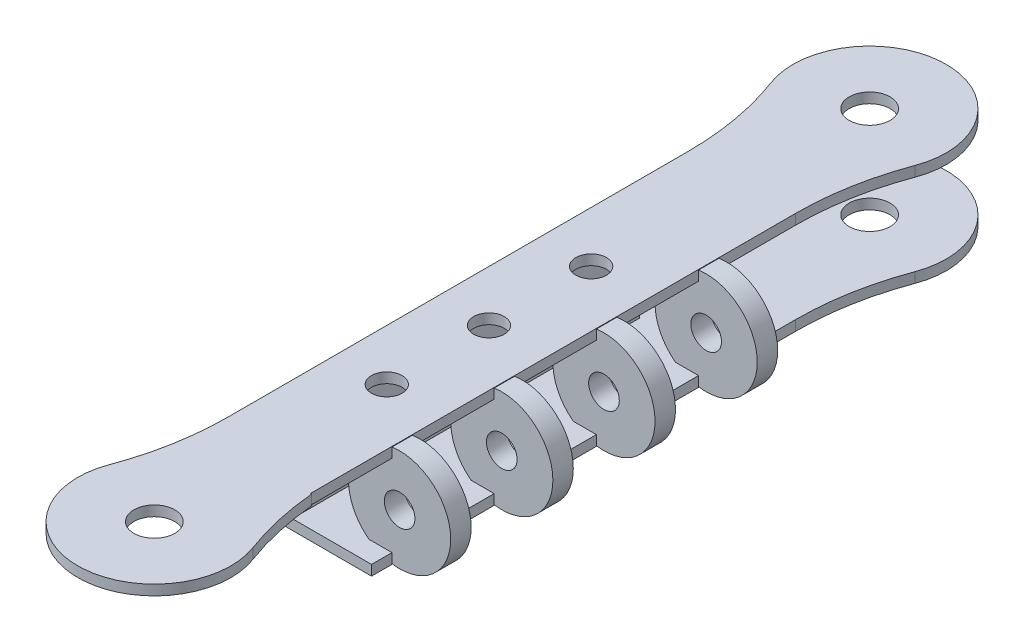
from build123d import *

# Parameters (mm, degrees)
BOSS_EXTRUDE1_DEPTH     = 10
CUT_EXTRUDE1_DEPTH      = 79.501592341
CUT_EXTRUDE1_DEPTH_BACK = 79.501592341
SKETCH2_R               = 2
CUT_EXTRUDE4_DEPTH      = 79.501592341
CUT_EXTRUDE4_DEPTH_BACK = 79.501592341
SKETCH5_W               = 10
SKETCH5_H               = 8
SKETCH3_R               = 5
BOSS_EXTRUDE2_DEPTH     = 40
CUT_EXTRUDE3_DEPTH      = 79.912926724
CUT_EXTRUDE3_DEPTH_BACK = 79.912926724
SKETCH4_W               = 4
SKETCH4_H               = 8
CUT_EXTRUDE5_DEPTH      = 80.176595509
CUT_EXTRUDE5_DEPTH_BACK = 5
SKETCH6_W               = 8
SKETCH6_H               = 7.999190419
SKETCH6_H_2             = 8
SKETCH6_H_3             = 8.000809581
SKETCH6_H_4             = 8.001619162
SKETCH7_W               = 5
SKETCH7_H               = 8
CUT_EXTRUDE6_DEPTH      = 60.390655831
CUT_EXTRUDE8_DEPTH      = 79.912926698
CUT_EXTRUDE8_DEPTH_BACK = 79.912926698
SKETCH9_R               = 1.5
CUT_EXTRUDE9_DEPTH      = 62.329030646
CUT_EXTRUDE9_DEPTH_BACK = 62.329030646
SKETCH10_R              = 1.5
SKETCH11_W              = 18
SKETCH11_H              = 9
CUT_EXTRUDE10_DEPTH     = 70.117653317
CUT_EXTRUDE11_DEPTH     = 6


with BuildPart() as part:
    # Sketch1 → Boss-Extrude1 (new body)
    with BuildSketch(Plane(origin=(0, 0, 0), x_dir=(1, 0, 0), z_dir=(0, 1, 0))):
        with BuildLine():
            Line((-5.254735448, -12.5), (-5.254735448, -57.5))
            ThreePointArc((-5.254735448, -57.5), (-5.702369539, -62.524085228), (-7.031169787, -67.389894366))
            ThreePointArc((-7.031169787, -67.389894366), (-7.381862008, -68.674061352), (-7.5, -70))
            ThreePointArc((-7.5, -70), (0, -77.5), (7.5, -70))
            ThreePointArc((7.5, -70), (7.381862008, -68.674061352), (7.031169787, -67.389894366))
            ThreePointArc((7.031169787, -67.389894366), (5.702369539, -62.524085228), (5.254735448, -57.5))
            Line((5.254735448, -57.5), (5.254735448, -12.5))
            ThreePointArc((5.254735448, -12.5), (5.702369539, -7.475914772), (7.031169787, -2.610105634))
            ThreePointArc((7.031169787, -2.610105634), (7.381862008, -1.325938648), (7.5, 0))
            ThreePointArc((7.5, 0), (0, 7.5), (-7.5, 0))
            ThreePointArc((-7.5, 0), (-7.381862008, -1.325938648), (-7.031169787, -2.610105634))
            ThreePointArc((-7.031169787, -2.610105634), (-5.702369539, -7.475914772), (-5.254735448, -12.5))
        make_face()
    extrude(amount=BOSS_EXTRUDE1_DEPTH)

    # Sketch2 → Cut-Extrude1 (cut, two sides: drawn at the far end of the back side and taken through both)
    with BuildSketch(Plane(origin=(0, 10, 0), x_dir=(1, 0, 0), z_dir=(0, 1, 0)).offset(-CUT_EXTRUDE1_DEPTH_BACK)):
        with Locations(Location((0, 0, 0), (0, 0, 270))):
            Circle(SKETCH2_R)
        with Locations(Location((0, -70, 0), (0, 0, 270))):
            Circle(SKETCH2_R)
    extrude(amount=CUT_EXTRUDE1_DEPTH + CUT_EXTRUDE1_DEPTH_BACK, mode=Mode.SUBTRACT)

    # Sketch5 → Cut-Extrude4 (cut, two sides: drawn at the far end of the back side and taken through both)
    with BuildSketch(Plane.XY.offset(-CUT_EXTRUDE4_DEPTH_BACK)):
        with Locations((2.5, 5)):
            Rectangle(SKETCH5_W, SKETCH5_H)
    extrude(amount=CUT_EXTRUDE4_DEPTH + CUT_EXTRUDE4_DEPTH_BACK, mode=Mode.SUBTRACT)

    # Sketch3 → Boss-Extrude2 (add)
    with BuildSketch(Plane.XY.offset(20)):
        with Locations((6, 5)):
            Circle(SKETCH3_R)
    extrude(amount=BOSS_EXTRUDE2_DEPTH)

    # Sketch4 → Cut-Extrude3 (cut, two sides: drawn at the far end of the back side and taken through both)
    with BuildSketch(Plane(origin=(0, 0, 0), x_dir=(1, 0, 0), z_dir=(0, 1, 0)).offset(-CUT_EXTRUDE3_DEPTH_BACK)):
        with Locations((7.254735448, -26)):
            Rectangle(SKETCH4_W, SKETCH4_H)
        with Locations((7.254735448, -36)):
            Rectangle(SKETCH4_W, SKETCH4_H)
        with Locations((7.254735448, -46)):
            Rectangle(SKETCH4_W, SKETCH4_H)
        with Locations((7.254735448, -56)):
            Rectangle(SKETCH4_W, SKETCH4_H)
    extrude(amount=CUT_EXTRUDE3_DEPTH + CUT_EXTRUDE3_DEPTH_BACK, mode=Mode.SUBTRACT)

    # Sketch6 → Cut-Extrude5 (cut, two sides: drawn at the far end of the back side and taken through both)
    with BuildSketch(Plane(origin=(5.254735448, 0, 0), x_dir=(0, 0, -1), z_dir=(1, 0, 0)).offset(-CUT_EXTRUDE5_DEPTH_BACK)):
        with Locations((-56, 4.99959521)):
            Rectangle(SKETCH6_W, SKETCH6_H)
        with Locations((-46, 5)):
            Rectangle(SKETCH6_W, SKETCH6_H_2)
        with Locations((-36, 5.000404791)):
            Rectangle(SKETCH6_W, SKETCH6_H_3)
        with Locations((-26, 5.000809581)):
            Rectangle(SKETCH6_W, SKETCH6_H_4)
    extrude(amount=CUT_EXTRUDE5_DEPTH + CUT_EXTRUDE5_DEPTH_BACK, mode=Mode.SUBTRACT)

    # Sketch7 → Cut-Extrude6 (cut, through all)
    with BuildSketch(Plane.XY.offset(20)):
        with Locations((-5, 5)):
            Rectangle(SKETCH7_W, SKETCH7_H)
    extrude(amount=-CUT_EXTRUDE6_DEPTH, mode=Mode.SUBTRACT)

    # Sketch9 → Cut-Extrude8 (cut, two sides: drawn at the far end of the back side and taken through both)
    with BuildSketch(Plane(origin=(0, 10, 0), x_dir=(1, 0, 0), z_dir=(0, 1, 0)).offset(-CUT_EXTRUDE8_DEPTH_BACK)):
        with Locations(Location((-0.254735448, -27, 0), (0, 0, 270))):
            Circle(SKETCH9_R)
        with Locations(Location((-0.254735448, -37, 0), (0, 0, 270))):
            Circle(SKETCH9_R)
        with Locations(Location((-0.254735448, -47, 0), (0, 0, 270))):
            Circle(SKETCH9_R)
    extrude(amount=CUT_EXTRUDE8_DEPTH + CUT_EXTRUDE8_DEPTH_BACK, mode=Mode.SUBTRACT)

    # Sketch10 → Cut-Extrude9 (cut, two sides: drawn at the far end of the back side and taken through both)
    with BuildSketch(Plane.XY.offset(52).offset(-CUT_EXTRUDE9_DEPTH_BACK)):
        with Locations((6, 5)):
            Circle(SKETCH10_R)
    extrude(amount=CUT_EXTRUDE9_DEPTH + CUT_EXTRUDE9_DEPTH_BACK, mode=Mode.SUBTRACT)

    # Sketch11 → Cut-Extrude10 (cut, through all)
    with BuildSketch(Plane.XY.offset(60)):
        with Locations((-0.335498684, 4.5)):
            Rectangle(SKETCH11_W, SKETCH11_H)
    extrude(amount=CUT_EXTRUDE10_DEPTH, mode=Mode.SUBTRACT)

    # Sketch12 → Cut-Extrude11 (cut)
    with BuildSketch(Plane.XY.offset(60)):
        Polygon((5.254735448, 0), (5.254735448, 1), (-2.5, 1), (-2.5, 9), (-5.364914213, 9), (-5.364914213, 0), align=None)
    extrude(amount=-CUT_EXTRUDE11_DEPTH, mode=Mode.SUBTRACT)


solid = part.part
